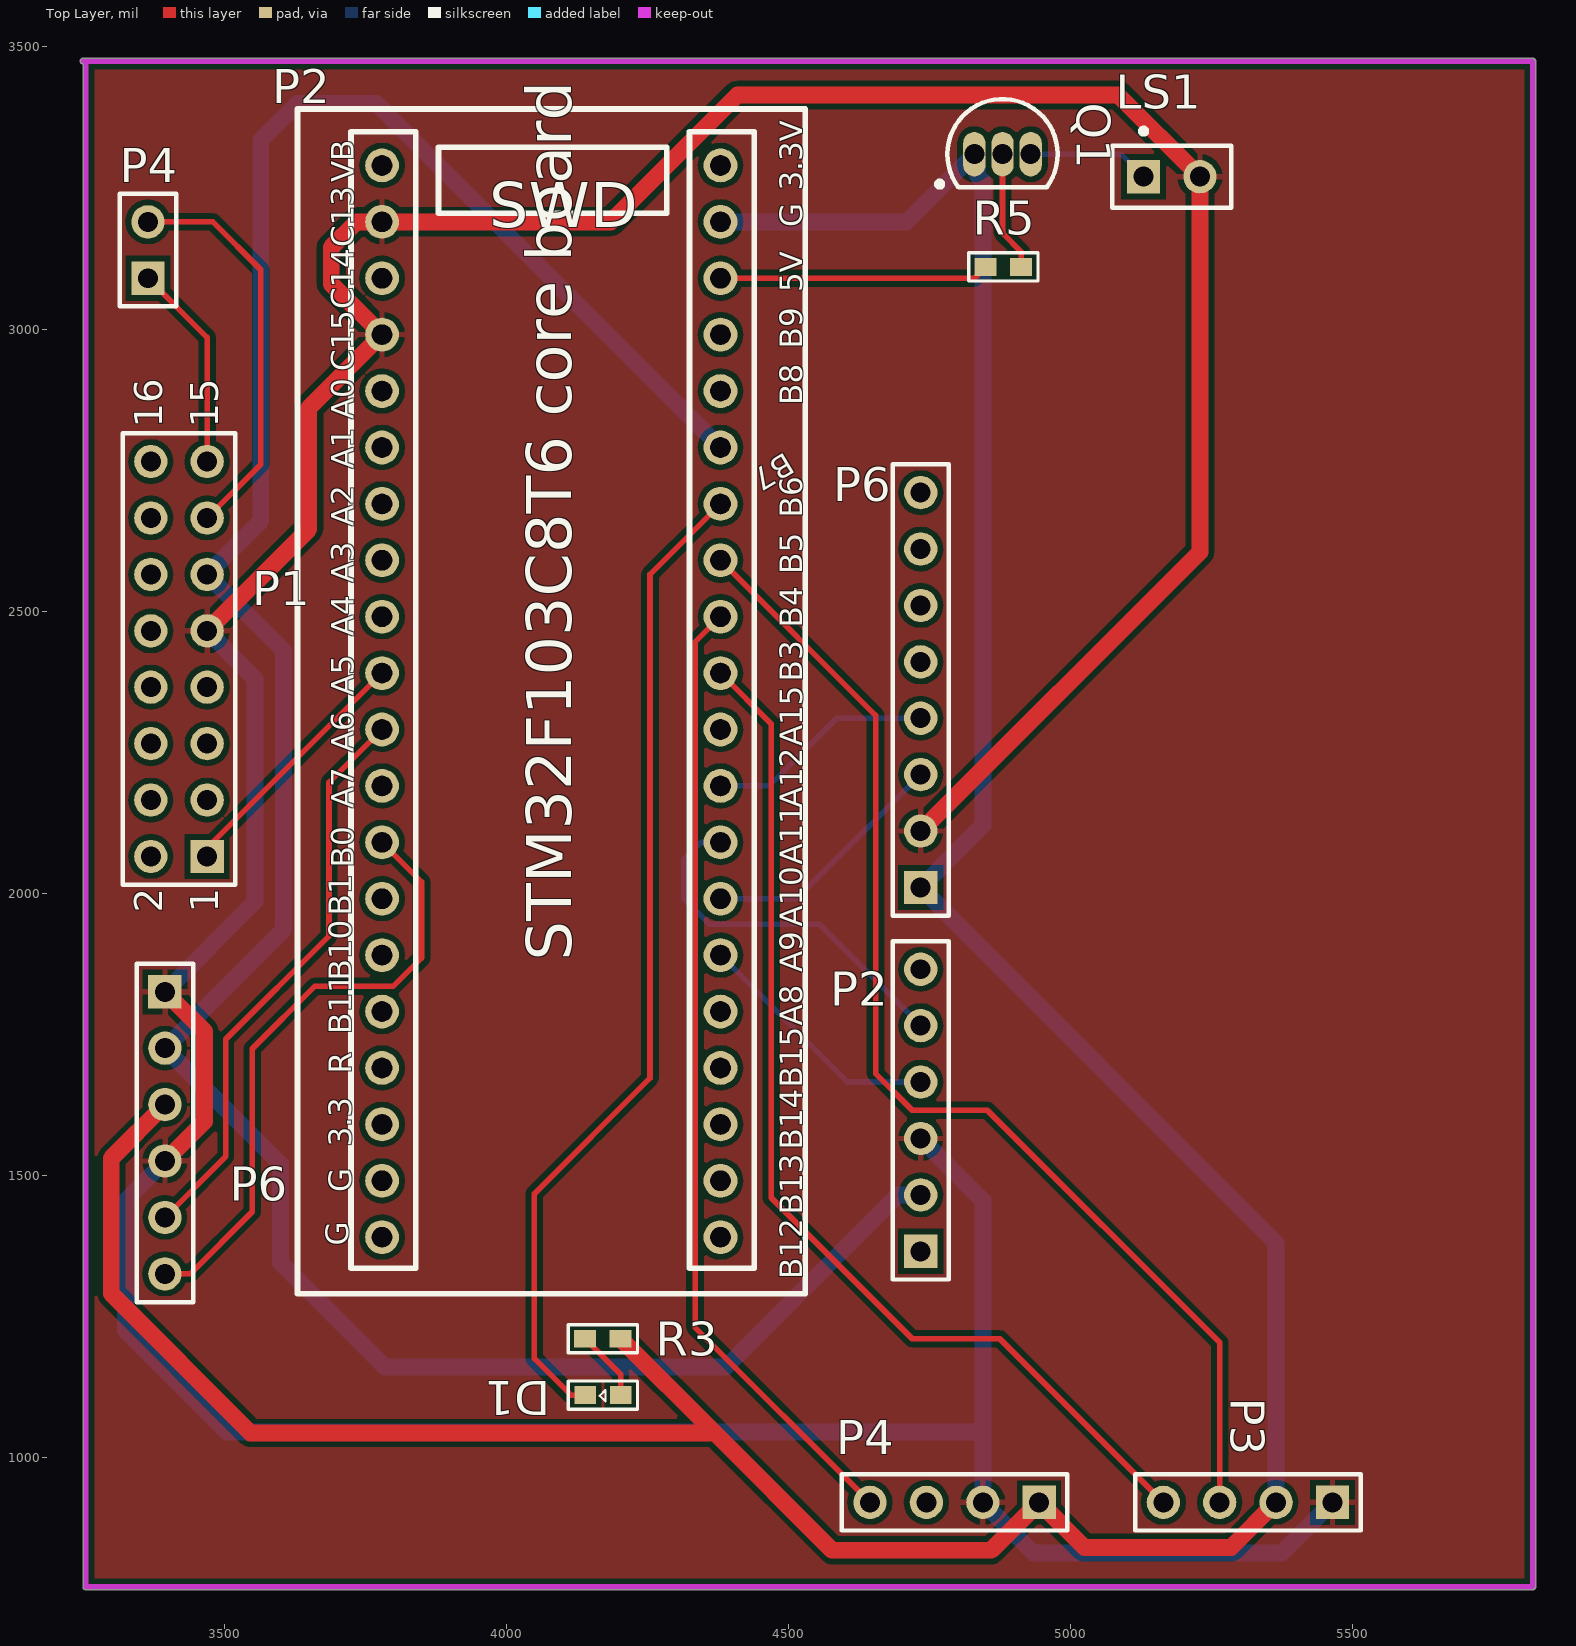
[diagram p0: Top Layer view]
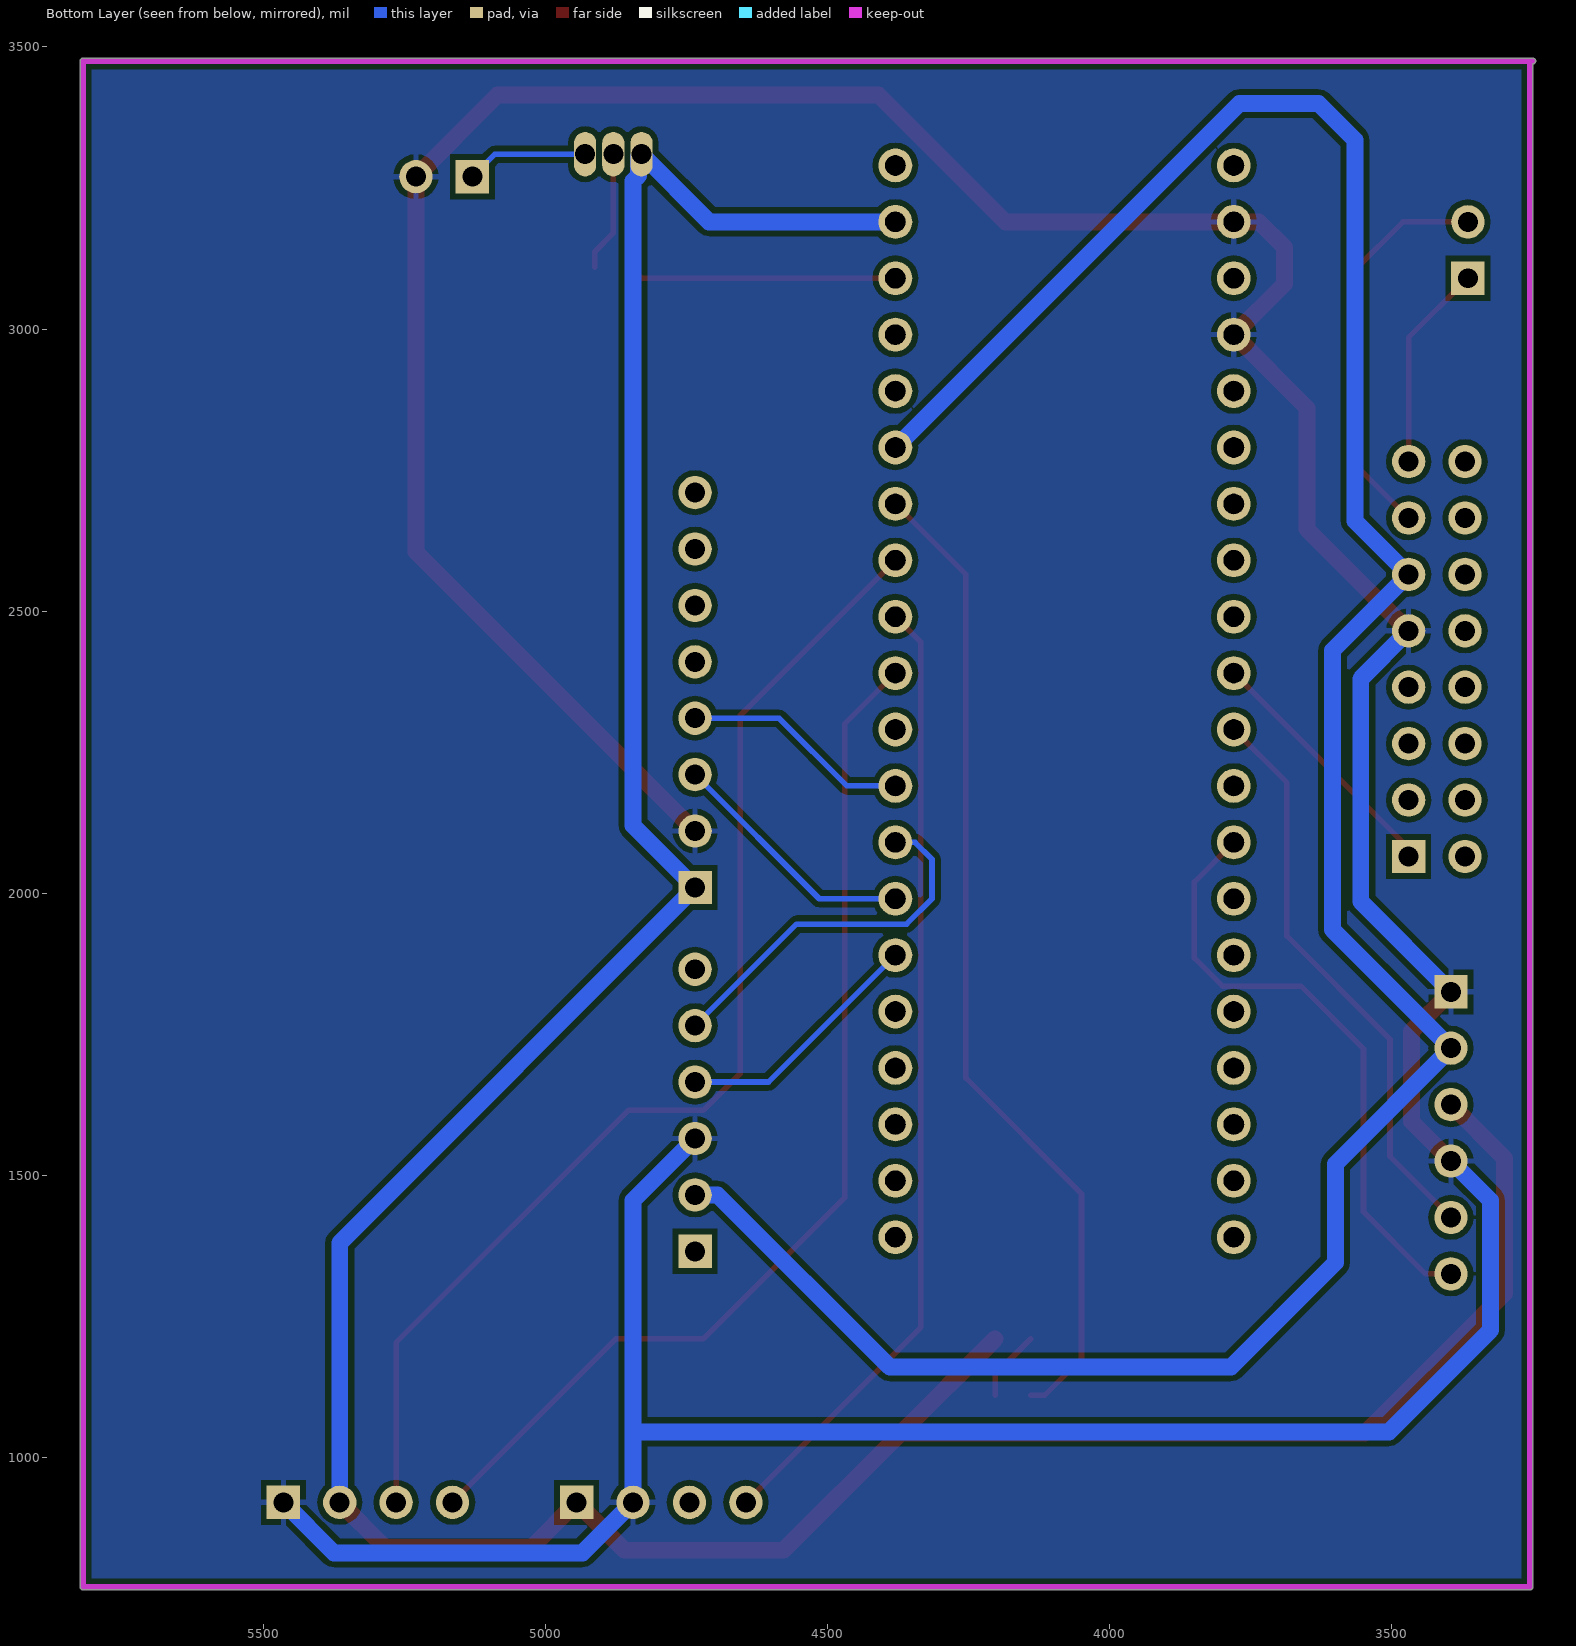
[diagram p1: Bottom Layer view, seen from below]
# Altium PCB MISC84382.PcbDoc
Units mil, origin at the board's own origin, x right, y up, seen from the top; angles counter-clockwise.
Board outline 2580.03 x 2715.03 mil, 2 copper layers (Top Layer, Bottom Layer); 13 components, 29 nets, 97 pads, 0 vias.

## Layer stack, top to bottom (the 12.6 mil dielectric is the usual default, probably not edited)
Top Solder: solder mask 0.4, Solder Resist, Dk 3.5
Top Layer: signal copper 1.4
Dielectric 1: dielectric 12.6, FR-4, Dk 4.8
Bottom Layer: signal copper 1.4
Bottom Solder: solder mask 0.4, Solder Resist, Dk 3.5

## Board outline
3249.99,770 3249.99,3469.99 cw(c3250,3475) 3250,3480.01 5820,3480.01 cw(c5820,3475) 5825.02,3475 5825.02,770 cw(c5820,770) 5820,764.99 3255,764.99 cw(c3255,770)

## Design rules (kind name [scope] priority, off if disabled: settings)
Clearance [All] p1: gap=10
MinimumSolderMaskSliver [All] p1: minsoldermaskwidth=0
PolygonConnect [All] p1: connectstyle=Relief reliefconductorwidth=10 reliefentries=4 polygonreliefangle="90 Angle" airgapwidth=10
RoutingVias [All] p1: holewidth=28 width=50 viastyle="Through Hole" minholewidth=28 minwidth=50 maxholewidth=28 maxwidth=50
SilkToSilkClearance [All] p1: silktosilkclearance=0
SilkToSolderMaskClearance [IsPad] p1: minsilkscreentomaskgap=0 clearancetoexposedcopper=TRUE
SolderMaskExpansion [All] p1: expansion=4
Width [All] p1: maxlimit=30 minlimit=10 preferedwidth=10
27 further rules are at their usual default settings.

## Classes and differential pairs
component class 电路图: D1 LS1 P1 P2 P3 P4 P6 Q1 R3 R5

## Components (designator, comment, footprint, x,y, rotation, side; value= is the part's Value field where it differs from the comment)
D1 "LED0" my0603LED 4202.99,1110 r180 top
LS1 "beef" PIN2 5130,3270 r0 top
P1 "JQ8900" HDR2X8 3470,2065 r90 top
P2 "JDY-31" HDR1X6 4735,1365 r90 top
P2 "STM32F103" STM32核心板 5281.5,2564 r0 top
P3 "0.96oled" HDR1X4 5465,920 r180 top
P4 "Photoresistor" HDR1X4 4945,920 r180 top
P4 "Speaker" HDR1X2 3365,3090 r90 top
P6 "MPU-6050" HDR1X8 4735,2010 r90 top
P6 "SIM900A" HDR1X6 3395,1825 r270 top
Q1 "8550" TO-92A 4880,3310 r270 top
R3 "510R" my0603 4140,1210 r0 top
R5 "1k" my0603 4850,3110 r0 top

## Footprints (in the part's own frame and the unit in brackets; to place one, negate y for a bottom-side part, rotate by r counter-clockwise, add the part's x,y. Pads: shape width x height; smd on the part's side, far side on the other; paste and mask are expansions set on the pad)
HDR1X2 [mm] "Connector; Header; 2 Position"
  rect 1.5x1.5 hole 0.9: 1(0,0)
  round 1.5 hole 0.9: 2(2.54,0)
  silkscreen extent -1.27,-1.27 3.81,1.27
HDR1X4 [mm] "Connector; Header; 4 Position"
  rect 1.5x1.5 hole 0.9: 1(0,0)
  round 1.5 hole 0.9: 2(2.54,0) 3(5.08,0) 4(7.62,0)
  silkscreen extent -1.27,-1.27 8.89,1.27
HDR1X6 [mm] "Connector; Header; 6 Position"
  rect 1.5x1.5 hole 0.9: 1(0,0)
  round 1.5 hole 0.9: 2(2.54,0) 3(5.08,0) 4(7.62,0) 5(10.16,0) 6(12.7,0)
  silkscreen extent -1.27,-1.27 13.97,1.27
HDR1X8 [mm] "Connector; Header; 8 Position"
  rect 1.5x1.5 hole 0.9: 1(0,0)
  round 1.5 hole 0.9: 2(2.54,0) 3(5.08,0) 4(7.62,0) 5(10.16,0) 6(12.7,0) 7(15.24,0) 8(17.78,0)
  silkscreen extent -1.27,-1.27 19.05,1.27
HDR2X8 [mm] "Connector; Header; 8x2 Position"
  rect 1.5x1.5 hole 0.9: 1(0,0)
  round 1.5 hole 0.9: 2(0,2.54) 3(2.54,0) 4(2.54,2.54) 5(5.08,0) 6(5.08,2.54) 7(7.62,0) 8(7.62,2.54) 9(10.16,0) 10(10.16,2.54) 11(12.7,0) 12(12.7,2.54) 13(15.24,0) 14(15.24,2.54) 15(17.78,0) 16(17.78,2.54)
  silkscreen extent -1.27,-1.27 19.05,3.81
my0603 [mm]
  rect 1x0.8 smd: 1(0,0) 2(1.6,0)
  silkscreen extent -0.76,-0.64 2.36,0.64
my0603LED [mm]
  rect 0.965x0.8 smd: 1(0,0) 2(1.6,0)
  silkscreen extent -0.76,-0.64 2.36,0.64
PIN2 [mm] "Photosensitive Diode; 2 Leads"
  rect 1.5x1.5 hole 0.9: 1(0,0)
  round 1.5 hole 0.9: 2(2.54,0)
  silkscreen extent -1.4,-1.4 3.94,2.17
STM32核心板 [mil]
  round 60 hole 36 slot 36.2 at 0 deg paste+0 mask+2: 1(-1501.5,726) 2(-1501.5,626) 3(-1501.5,526) 4(-1501.5,426) 5(-1501.5,326) 6(-1501.5,226) 7(-1501.5,126) 8(-1501.5,26) 9(-1501.5,-74) 10(-1501.5,-174) 11(-1501.5,-274) 12(-1501.5,-374) 13(-1501.5,-474) 14(-1501.5,-574) 15(-1501.5,-674) 16(-1501.5,-774) 17(-1501.5,-874) 18(-1501.5,-974) 19(-1501.5,-1074) 20(-1501.5,-1174) 21(-901.5,-1174) 22(-901.5,-1074) 23(-901.5,-974) 24(-901.5,-874) 25(-901.5,-774) 26(-901.5,-674) 27(-901.5,-574) 28(-901.5,-474) 29(-901.5,-374) 30(-901.5,-274) 31(-901.5,-174) 32(-901.5,-74) 33(-901.5,26) 34(-901.5,126) 35(-901.5,226) 36(-901.5,326) 37(-901.5,426) 38(-901.5,526) 39(-901.5,626) 40(-901.5,726)
  silkscreen extent -1652,-1274 -752,826
TO-92A [mm] "TO, Flat Index; 3 In-Line, Axial Leads; Body Dia. 4.5mm; Leads 0.51 x 0.48 mm (max)"
  oval 2x1 hole 0.9: 1(0,-1.27) 2(0,0) 3(0,1.27)
  silkscreen extent -2.48,-2.95 1.5,2.48, body extent -2.48,-2.5 1.5,2.5, height 6.86

## Part data
D1: "Typical INFRARED GaAs LED"
LS1: library part BEEP, "Buzzer"
P1: library part "Header 8X2", "Header, 8-Pin, Dual row"
P2 P6: library part "Header 6", "Header, 6-Pin"
P2: library part "Header 20X2", "Header, 20-Pin, Dual row"
P3: library part "Header 4", "Header, 4-Pin"
P4: library part Component_1
P4: library part "Header 2", "Header, 2-Pin"
P6: library part "Header 8", "Header, 8-Pin"
Q1: library part 2N3906, "PNP General Purpose Amplifier"
R3: library part R
R5: library part R, "SMD resistor"

## Nets (pads, with @x,y where several pads share a name; then routed paths per layer and width w, separated by ;. In a path a pad name is that pad's centre, name@x,y a point inside that pad or via, vN(x,y) a via of type N, cw(c..) or ccw(c..) an arc to the next point about the centre after c; other vN are vias at no path point)
3V3: P2.39 P3.2 P4.1@4945,920 P6.1@4735,2010 P6.3@3395,1625 Q1.1 R3.2 | length 6167.9
  Top Layer w30: P6.3@3395,1625 3300,1530 3300,1290 3547.01,1042.99 4370,1042.99 ; R3.2 4370,1042.99 ; P3.2 5285,840 5025,840 4945,920 4860,835 4577.99,835 4370,1042.99
  Bottom Layer w30: P2.39 4710,3190 Q1.1 4835.31,3304.68 4835.31,3271.81 4845,3262.12 4845,2120 4735,2010 5365,1380 P3.2
5V: 
+5V: P1.11 P2.2@4735,1465 P2.35 P6.2@3395,1725 | length 4689.7
  Bottom Layer w30: P2.35 3770,3400 3630,3400 3565,3335 3565,2660 P1.11 3605,2430 3605,1935 3395,1725 3600,1520 3600,1345 3785,1160 4390,1160 4695,1465 P2.2@4735,1465
DAC: P1.2
GND: LS1.2 P1.9 P2.2@3780,3190 P2.3@4735,1565 P2.4@3780,2990 P3.1 P4.2@4845,920 P6.1@3395,1825 P6.2@4735,2110 P6.4@3395,1525 | length 8330.8
  Top Layer w30: P6.4@3395,1525 3465,1595 3465,1755 P6.1@3395,1825 ; P1.9 3650,2645 3650,2860 3780,2990 3690,3080 3690,3145 3735,3190 3780,3190 4185,3190 4410,3415 5085,3415 LS1.2 5230,2605 P6.2@4735,2110
  Bottom Layer w30: P6.4@3395,1525 3325,1455 3325,1225 3505,1045 4845,1045 ; P6.1@3395,1825 3555,1985 3555,2380 P1.9 ; P2.3@4735,1565 4845,1455 4845,1045 ; P3.1 5375,830 4935,830 4845,920 4845,1045
IO1: P1.4
IO2: P1.6
IO3: P1.8
IO4: P1.10
IO5: P1.12
IO6: P1.14
IO7: P1.16
NetD1_1: D1.1 R3.1 | length 126.1
  Top Layer w10: R3.1 4202.99,1147.01 D1.1
NetLS1_1: LS1.1 Q1.3 | length 216.6
  Bottom Layer w10: Q1.3 5090,3310 LS1.1
NetQ1_2: Q1.2 R5.2 | length 213.7
  Top Layer w10: Q1.2 4880,3170 4913,3137 R5.2
PA0: P2.32 P4.4 | length 1717
  Top Layer w10: P2.32 4335,2445 4335,1230 P4.4
PA2: P2.5@4735,1765 P2.28 | length 660.6
  Bottom Layer w10: P2.28 4345,2090 4315,2060 4315,1990 4360,1945 4555,1945 P2.5@4735,1765
PA3: P2.4@4735,1665 P2.26 | length 448.2
  Bottom Layer w10: P2.26 4605,1665 P2.4@4735,1665
PA9: P2.11 P6.5@3395,1425 | length 1024.5
  Top Layer w10: P6.5@3395,1425 3503,1533 3503,1741 3686,1924 3686,2196 P2.11
PA10: P2.13 P6.6@3395,1325 | length 1090.2
  Top Layer w10: P6.6@3395,1325 3440,1325 3550,1435 3550,1724 3661,1835 3800,1835 3850,1885 3850,2020 P2.13
PB6: P2.27 P6.3@4735,2210 | length 446.1
  Bottom Layer w10: P2.27 4515,1990 P6.3@4735,2210
PB7: P2.29 P6.4@4735,2310 | length 404.7
  Bottom Layer w10: P2.29 4466,2190 4586,2310 P6.4@4735,2310
PB11: P1.1 P2.10 | length 453.4
  Top Layer w10: P1.1 3470,2080 P2.10
PC13: P2.38 R5.1 | length 478.3
  Top Layer w10: P2.38 4830,3090 R5.1
PC15: D1.2 P2.34 | length 1768.6
  Top Layer w10: D1.2 4115,1110 4050,1175 4050,1467 4255,1672 4255,2565 P2.34
SCL: P2.33 P3.3 | length 2114.5
  Top Layer w10: P2.33 4655,2315 4655,1680 4720,1615 4853,1615 5265,1203 P3.3
SDA: P2.31 P3.4 | length 1886
  Top Layer w10: P2.31 4470,2300 4470,1460 4720,1210 4875,1210 P3.4
SPK+: P1.15 P4.1@3365,3090 | length 368.5
  Top Layer w10: P4.1@3365,3090 3470,2985 P1.15
SPK-: P1.13 P4.2@3365,3190 | length 714.6
  Top Layer w10: P4.2@3365,3190 3480,3190 3565,3105 3565,2760 P1.13
pads on no net: P1.3 P1.5 P1.7 P2.1 P2.3@3780,3090 P2.5@3780,2890 P2.6 P2.7 P2.8 P2.9 P2.12 P2.14 P2.15 P2.16 P2.17 P2.18 P2.19 P2.20 P2.21 P2.22 P2.23 P2.24 P2.25 P2.30 P2.36 P2.37 P2.40 P4.3 P6.5@4735,2410 P6.6@4735,2510 P6.7 P6.8

## Polygon pours and split planes (outlines as drawn)
GND on Top Layer "Top Layer-No Net" (solid, remove dead copper, pour order 4): 2790,3760 2820,3730 6705,3730 6705,365 6460,120 6050,530 3320,530 3020,530
GND on Bottom Layer "Top Layer-No Net" (solid, remove dead copper, pour order 6): 2625,3960 2845,3740 7300,3740 7300,1160 6510,370 6470,410 2095,410

## Keep-outs
Keep-Out Layer:
  lines w10: 3250,3475 5275,3475 ; 3255,3475 3255,1275 3255,770 3285,770 5820,770 5820,3475 5435,3475 ; 5225,3475 5450,3475